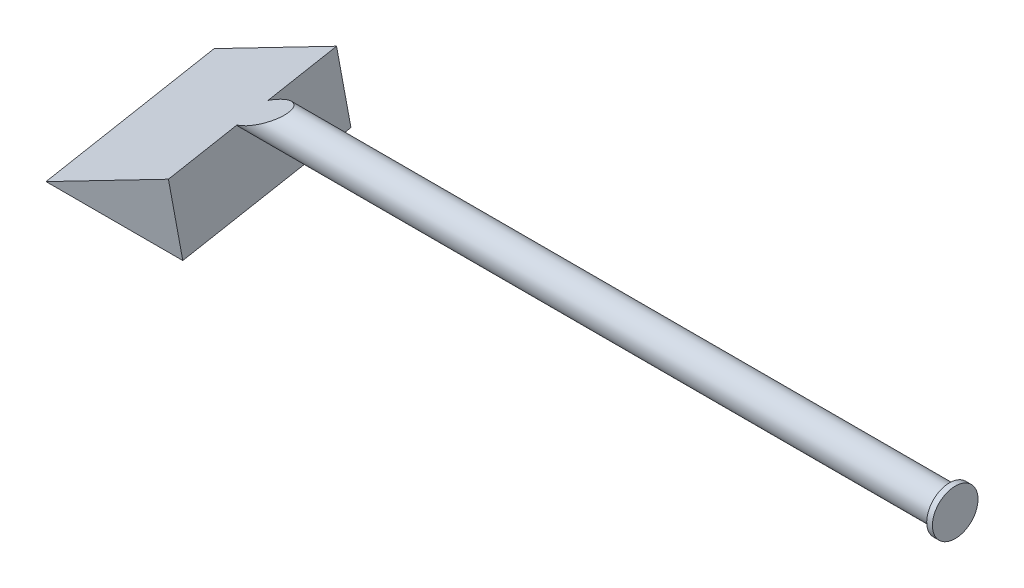
SolidWorks part; units mm, degrees
ref_plane "Front Plane" through (0, 0, 0) normal (0, 0, 1) x (1, 0, 0)
ref_plane "Top Plane" through (0, 0, 0) normal (0, 1, 0) x (1, 0, 0)
ref_plane "Right Plane" through (0, 0, 0) normal (1, 0, 0) x (0, 0, -1)
sketch "Sketch1" plane through (0, 0, 0) normal (0, 0, 1) x (1, 0, 0)
  line L0 (-22, 0) -> (96, 0) construction
  line L1 (-38, 0) -> (-22, 0) construction
  line L2 (-38, 0) -> (-38, 3)
  line L3 (-38, 3) -> (84.5, 3)
  line L4 (84.5, 3) -> (84.5, 4)
  line L5 (84.5, 4) -> (85.5, 4)
  line L6 (85.5, 4) -> (85.5, 0)
  line L7 (85.5, 4) -> (96, 4) construction
  line L9 (-38, 0) -> (-38, -1)
  line L10 (-24.6667, 3) -> (-24.6667, 2.7)
  line L11 (-32.5, -5) -> (-27.5, -5)
  line L12 (-32.5, -5) -> (-32.5, 5)
  line L13 (-32.5, 5) -> (-27.5, 5)
  line L14 (-27.5, -5) -> (-27.5, 5)
  line L15 (-32.5, -5) -> (-27.5, 5) construction
  line L16 (-32.5, 5) -> (-27.5, -5) construction
  line L17 (-22, 2.5) -> (-17, 2.5)
  line L18 (-22, 2.5) -> (-22, -2.5)
  line L19 (-22, -2.5) -> (-17, -2.5)
  line L20 (-17, 2.5) -> (-17, -2.5)
  line L21 (-24.6667, 2.7) -> (-22, 2.7)
  line L22 (-22, 2.7) -> (-22, 3)
  point P4 (136, 0)
  point P6 (2, 0)
  point P14 (-30, 0)
  point P20 (-17, 0)
  dimension "N" = 22
  dimension "H" = 16
  dimension "行程" = 40
  dimension "C1" = 10.5
  dimension "D2" = 1
  dimension "D3" = 1
  dimension "K" = 6
  dimension "D5" = 2.6667
  dimension "KM" = 1
  dimension "J" = 5
  dimension "T" = 10
  dimension "I" = 17
  dimension "Y" = 5
  dimension "D6" = 0.3
  dimension "A4+行程" = 134
  dimension "A6" = 94
sketch "Sketch2" plane through (0, 0, 0) normal (0, 0, 1) x (1, 0, 0)
  line L0 (-38, 0) -> (-38, 3) construction
  line L1 (-38, 0) -> (-22, 0) construction
  line L2 (-38, 3) -> (84.5, 3) construction
  line L3 (-24.6667, 3) -> (-24.6667, 2.7) construction
  line L4 (-24.6667, 2.7) -> (-22, 2.7) construction
  line L5 (-22, 2.7) -> (-22, 3) construction
  line L6 (84.5, 3) -> (84.5, 4) construction
  line L7 (84.5, 4) -> (85.5, 4) construction
  line L8 (85.5, 4) -> (85.5, 0) construction
  line L9 (-22, 0) -> (96, 0) construction
  line L10 (-38, 0) -> (-38, 2.475)
  line L11 (-38, 0) -> (-22, 0)
  line L12 (-37.475, 3) -> (-24.6667, 3)
  line L13 (-24.6667, 3) -> (-24.6667, 2.7)
  line L14 (-24.6667, 2.7) -> (-22, 2.7)
  line L15 (-22, 2.7) -> (-22, 3)
  line L16 (84.5, 3) -> (84.5, 4)
  line L17 (84.5, 4) -> (85.5, 4)
  line L18 (85.5, 4) -> (85.5, 0)
  line L19 (-22, 0) -> (85.5, 0)
  line L20 (-22, 3) -> (84.5, 3)
  line L21 (-38, 2.475) -> (-37.475, 3)
revolve "Revolve1" add sketch "Sketch2" angle 360 about L19
sketch "Sketch3" plane through (0, 0, 0) normal (1, 0, 0) x (0, 0, -1)
  line L1 (0, 5) -> (-4.3301, 2.5)
  line L2 (-4.3301, 2.5) -> (-4.3301, -2.5)
  line L3 (-4.3301, -2.5) -> (0, -5)
  line L4 (0, -5) -> (4.3301, -2.5)
  line L5 (4.3301, -2.5) -> (4.3301, 2.5)
  line L6 (4.3301, 2.5) -> (0, 5)
  circle A0 centre (0, 0) radius 4.3301 construction
sketch "Sketch5" plane through (-38, 0, 0) normal (-1, 0, 0) x (0, 0, 1)
  circle A0 centre (0, 0) radius 3 construction
  circle A1 centre (0, 0) radius 3
curve "Helix/Spiral1" pitch 1 height 12.6667 turns 12.6667
sketch "Sketch6" plane through (0, 0, 0) normal (0, 0, 1) x (1, 0, 0)
  line L1 (-37.875, 2.5714) -> (-37.5038, 3.2143)
  line L2 (-37.5038, 3.2143) -> (-38.2462, 3.2143)
  line L3 (-38.2462, 3.2143) -> (-37.875, 2.5714)
  circle A0 centre (-37.875, 3) radius 0.2143 construction
  dimension "D1" = 0.4286
sweep "Cut-Sweep1" cut profiles "Sketch6" path "Helix/Spiral1"
sketch "Sketch7" plane through (-22, 0, 0) normal (-1, 0, 0) x (0, 0, 1)
  line L0 (0, 0) -> (3, 0) construction
  line L1 (0, 0) -> (-3, 0) construction
  circle A0 centre (0, 0) radius 3 construction
  point P6 (2.5, 0)
  point P8 (-2.5, 0)
  dimension "D1" = 0.5
  dimension "D2" = 0.5
sketch "Sketch8" plane through (0, 0, 0) normal (0, 0, 1) x (1, 0, 0)
  line L0 (-22, 2.5) -> (-17, 2.5) construction
  line L1 (-22, 2.5) -> (-22, -2.5) construction
  line L2 (-22, -2.5) -> (-17, -2.5) construction
  line L3 (-17, 2.5) -> (-17, -2.5) construction
  line L4 (-22, 2.5) -> (-17, 2.5)
  line L5 (-22, 2.5) -> (-22, -2.5)
  line L6 (-22, -2.5) -> (-17, -2.5)
  line L7 (-17, 2.5) -> (-17, -2.5)
extrude "Y1" cut sketch "Sketch8" along normal up to vertex (3 mm away) from vertex at 2.5 starting at point (-22, 0, 2.5)
sketch "Sketch9" plane through (0, 0, 0) normal (0, 0, 1) x (1, 0, 0)
  line L0 (-17, 2.5) -> (-17, -2.5) construction
  line L1 (-22, 2.5) -> (-17, 2.5) construction
  line L2 (-22, -2.5) -> (-17, -2.5) construction
  line L3 (-22, 2.5) -> (-22, -2.5) construction
  line L4 (-17, 2.5) -> (-17, -2.5)
  line L5 (-22, 2.5) -> (-17, 2.5)
  line L6 (-22, -2.5) -> (-17, -2.5)
  line L7 (-22, 2.5) -> (-22, -2.5)
extrude "Y" cut sketch "Sketch9" against normal up to vertex (3 mm away) from vertex at -2.5 starting at point (-22, 0, -2.5)
scale "Scale 1" bodies to scale 106 scale about origin uniform scaling yes scale factor 0.5
sketch "Sketch10" plane through (-19, 0, 0) normal (-1, 0, 0) x (0, 0, 1)
  circle A0 centre (0, 0) radius 1.5
  dimension "D1" = 3
extrude "Boss-Extrude2" add sketch "Sketch10" against normal blind 12
sketch "Sketch11" plane through (-19, 0, 0) normal (-1, 0, 0) x (0, 0, 1)
  line L4 (-8.739, -6.0108) -> (-6.0108, 8.739)
  line L5 (6.0108, -8.739) -> (-8.739, -6.0108)
  line L6 (8.739, 6.0108) -> (6.0108, -8.739)
  line L7 (-6.0108, 8.739) -> (8.739, 6.0108)
extrude "Boss-Extrude3" add sketch "Sketch11" along normal blind 12
sketch "Sketch12" plane through (0, 1.3641, -7.3749) normal (0, 0.1819, -0.9833) x (-1, 0, 0)
  line L0 (5.0192, 7.5) -> (31, -7.5)
  line L1 (31, -7.5) -> (31, 7.5)
  line L2 (31, 7.5) -> (5.0192, 7.5)
  line L3 (31, -7.5) -> (19, -7.5) construction
  dimension "D1" = 30
extrude "Cut-Extrude1" cut sketch "Sketch12" against normal blind 49
